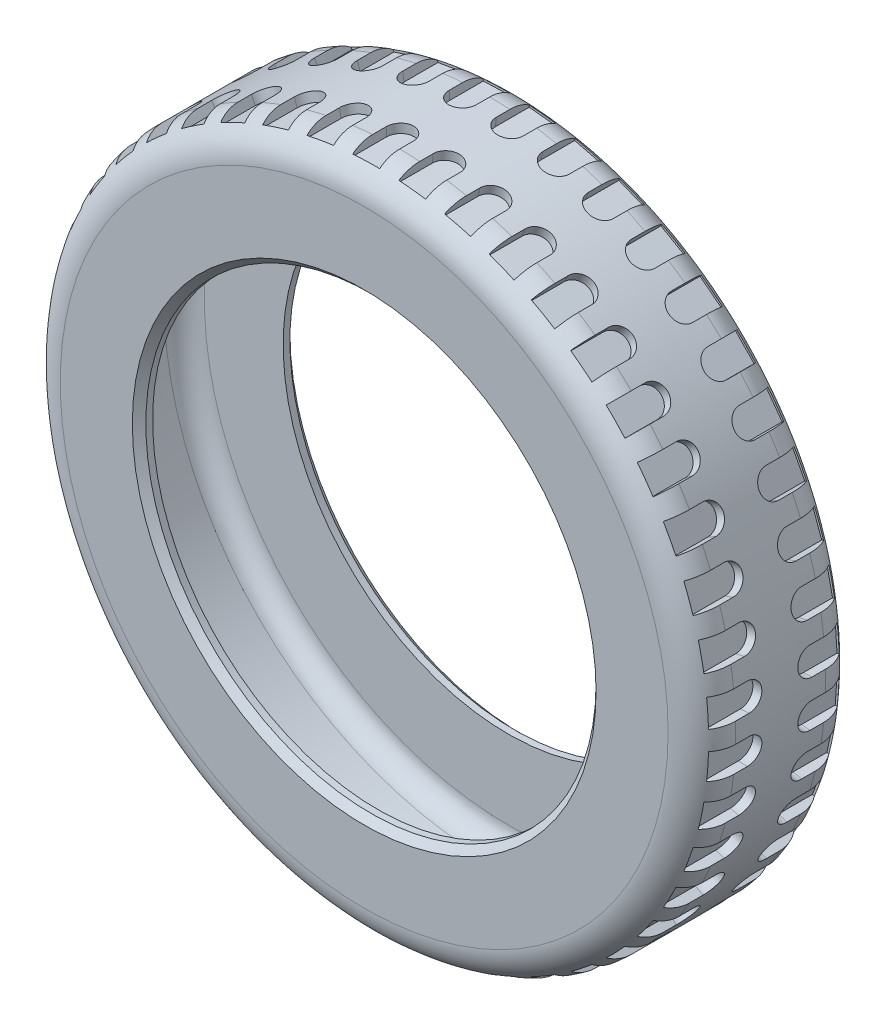
SolidWorks part; units mm, degrees
ref_plane "Front Plane" through (0, 0, 0) normal (0, 0, 1) x (1, 0, 0)
ref_plane "Top Plane" through (0, 0, 0) normal (0, 1, 0) x (1, 0, 0)
ref_plane "Right Plane" through (0, 0, 0) normal (1, 0, 0) x (0, 0, -1)
sketch "Sketch1" plane through (0, 0, 0) normal (0, 0, 1) x (1, 0, 0)
  circle A0 centre (0, 0) radius 5
  circle A1 centre (0, 0) radius 7.5
  dimension "D1" = 10
  dimension "D2" = 15
extrude "Boss-Extrude1" add sketch "Sketch1" along normal mid plane 3.5
fillet "Fillet1" radius 0.75 2 edges at (7.5, 0, 1.75) (7.5, 0, -1.75)
shell "Shell1" thickness 0.3
chamfer "Chamfer1" distance 0.15 angle 45 2 edges at (5, 0, -1.75) (5, 0, 1.75)
sketch "Sketch2" plane through (0, 0, 0) normal (1, 0, 0) x (0, 0, -1)
  line L0 (-0.7, 0.3) -> (-1.45, 0.3)
  line L1 (-1.45, 0.3) -> (-1.45, -0.3)
  line L2 (-1.45, -0.3) -> (-0.7, -0.3)
  line L4 (-1.75, 6.75) -> (-1.75, -6.75) construction
  line L5 (0, 0) -> (0, 3.1473) construction
  line L6 (1.45, -0.3) -> (0.7, -0.3)
  line L7 (1.45, 0.3) -> (1.45, -0.3)
  line L8 (0.7, 0.3) -> (1.45, 0.3)
  arc A0 (-0.7, 0.3) -> (-0.7, -0.3) centre (-0.7, 0) cw
  arc A1 (0.7, 0.3) -> (0.7, -0.3) centre (0.7, 0) ccw
  dimension "D1" = 0.3
  dimension "D2" = 0.7
  dimension "D3" = 0.3
extrude "Cut-Extrude1" cut sketch "Sketch2" along normal blind 7.5 and the other way blind 0.5 from offset 14.8 offset against normal yes
pattern_circular "CirPattern1" count 45 over 360 about axis through (0, 0, 0) along (0, 0, 1) of "Cut-Extrude1"
